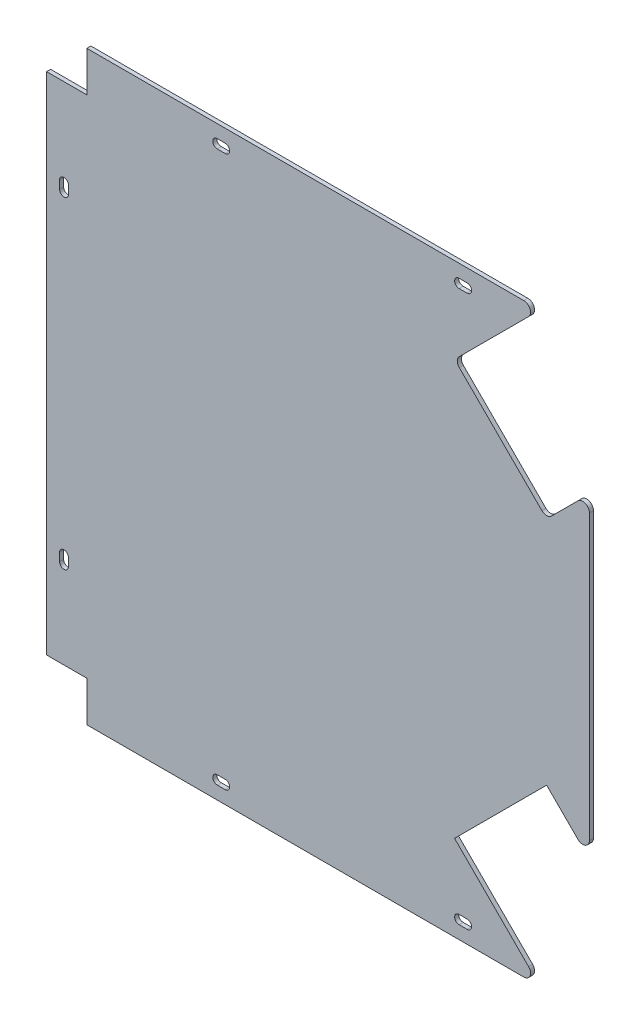
from build123d import *

# Parameters (mm, degrees)
SKETCH_1_W          = 440
SKETCH_1_H          = 436
EXTRUDE_1_DEPTH     = 3
SKETCH_2_W          = 30
SKETCH_2_H          = 30
CUT_EXTRUDE_1_DEPTH = 10
CUT_EXTRUDE_2_DEPTH = 10
CUT_EXTRUDE_3_DEPTH = 10
EXTRUDE_2_DEPTH     = 3
FILLET_1_R          = 5
CUT_EXTRUDE_4_DEPTH = 10


with BuildPart() as part:
    # 草图1 → 凸台-拉伸1 (new body)
    with BuildSketch(Plane.XY):
        Rectangle(SKETCH_1_W, SKETCH_1_H)
    extrude(amount=EXTRUDE_1_DEPTH)

    # 草图2 → 切除-拉伸1 (cut)
    with BuildSketch(Plane.XY.offset(3)):
        with Locations((-205, -203)):
            Rectangle(SKETCH_2_W, SKETCH_2_H)
        with Locations((-205, 203)):
            Rectangle(SKETCH_2_W, SKETCH_2_H)
    extrude(amount=-CUT_EXTRUDE_1_DEPTH, mode=Mode.SUBTRACT)

    # 草图3 → 切除-拉伸2 (cut)
    with BuildSketch(Plane.XY.offset(3)):
        Polygon((220, 218), (20, 218), (220, 18), align=None)
        Polygon((220, -218), (220, -18), (20, -218), align=None)
    extrude(amount=-CUT_EXTRUDE_2_DEPTH, mode=Mode.SUBTRACT)

    # 草图4 → 切除-拉伸3 (cut)
    with BuildSketch(Plane.XY.offset(3)):
        Polygon((220, 18), (184, 54), (184, -54), (220, -18), align=None)
    extrude(amount=-CUT_EXTRUDE_3_DEPTH, mode=Mode.SUBTRACT)

    # 草图5 → 凸台-拉伸2 (add)
    with BuildSketch(Plane.XY.offset(3)):
        Polygon((20, 218), (83.639610307, 154.360389693), (147.279220614, 218), align=None)
        Polygon((152.180194847, 85.819805153), (184, 54), (184, 117.639610307), align=None)
    extrude_2 = extrude(amount=-EXTRUDE_2_DEPTH)

    # 镜向1: 凸台-拉伸2 across plane
    add(extrude_2.mirror(Plane.ZX))

    # 圆角1
    fillet_1_edges = [part.edges().sort_by_distance(p)[0] for p in [
        (83.639610307, 154.360389693, 1.5),
        (147.279220614, 218, 1.5),
        (184, 117.639610307, 1.5),
        (152.180194847, 85.819805153, 1.5),
        (147.279220614, -218, 1.5),
        (184, -117.639610307, 1.5),
    ]]
    fillet(fillet_1_edges, radius=FILLET_1_R)

    # 草图6 → 切除-拉伸4 (cut)
    with BuildSketch(Plane(origin=(0, 0, 0), x_dir=(-1, 0, 0), z_dir=(0, 0, -1))):
        with BuildLine():
            Line((-93, 208.3), (-87, 208.3))
            ThreePointArc((-87, 208.3), (-83.7, 205), (-87, 201.7))
            Line((-87, 201.7), (-93, 201.7))
            ThreePointArc((-93, 201.7), (-96.3, 205), (-93, 208.3))
        make_face()
        with BuildLine():
            Line((87, 208.3), (93, 208.3))
            ThreePointArc((93, 208.3), (96.3, 205), (93, 201.7))
            Line((93, 201.7), (87, 201.7))
            ThreePointArc((87, 201.7), (83.7, 205), (87, 208.3))
        make_face()
        with BuildLine():
            Line((210.3, 123), (210.3, 117))
            ThreePointArc((210.3, 117), (207, 113.7), (203.7, 117))
            Line((203.7, 117), (203.7, 123))
            ThreePointArc((203.7, 123), (207, 126.3), (210.3, 123))
        make_face()
        with BuildLine():
            Line((210.3, -117), (210.3, -123))
            ThreePointArc((210.3, -123), (207, -126.3), (203.7, -123))
            Line((203.7, -123), (203.7, -117))
            ThreePointArc((203.7, -117), (207, -113.7), (210.3, -117))
        make_face()
        with BuildLine():
            Line((93, -208.3), (87, -208.3))
            ThreePointArc((87, -208.3), (83.7, -205), (87, -201.7))
            Line((87, -201.7), (93, -201.7))
            ThreePointArc((93, -201.7), (96.3, -205), (93, -208.3))
        make_face()
        with BuildLine():
            Line((-93, -201.7), (-87, -201.7))
            ThreePointArc((-87, -201.7), (-83.7, -205), (-87, -208.3))
            Line((-87, -208.3), (-93, -208.3))
            ThreePointArc((-93, -208.3), (-96.3, -205), (-93, -201.7))
        make_face()
    extrude(amount=-CUT_EXTRUDE_4_DEPTH, mode=Mode.SUBTRACT)


solid = part.part
